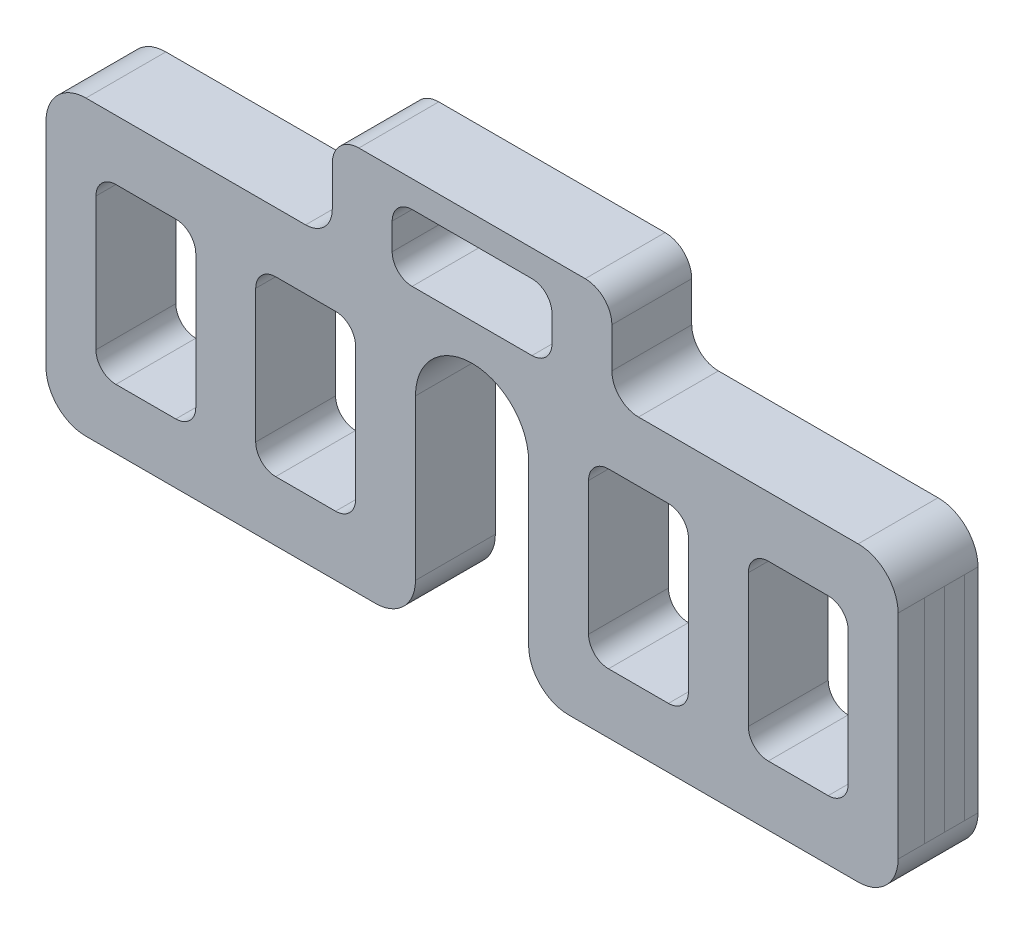
SolidWorks part; units mm, degrees
material "Q235-A"
ref_plane "Front Plane" through (0, 0, 0) normal (0, 0, 1) x (1, 0, 0)
ref_plane "Top Plane" through (0, 0, 0) normal (0, 1, 0) x (1, 0, 0)
ref_plane "Right Plane" through (0, 0, 0) normal (1, 0, 0) x (0, 0, -1)
sketch "Sketch1" plane through (0, 0, 0) normal (0, 0, 1) x (1, 0, 0)
  line L0 (0, -245) -> (0, 245) construction
  line L1 (42.5, 0) -> (320, 0)
  line L3 (45, 220) -> (-45, 220)
  line L4 (60, 235) -> (60, 255)
  line L5 (320, 0) -> (320, 220)
  line L6 (320, 220) -> (125, 220)
  line L7 (42.5, 0) -> (42.5, 150)
  line L8 (-42.5, 0) -> (-42.5, 150)
  line L9 (-320, 0) -> (-320, 220)
  line L10 (45, 270) -> (-45, 270)
  line L11 (-125, 220) -> (-320, 220)
  line L12 (-105, 240) -> (-105, 270)
  line L13 (-42.5, 0) -> (-320, 0)
  line L14 (105, 240) -> (105, 270)
  line L15 (-85, 290) -> (85, 290)
  line L16 (-60, 235) -> (-60, 255)
  line L17 (60, 220) -> (-60, 270) construction
  line L18 (60, 270) -> (-60, 220) construction
  arc A0 (-60, 235) -> (-45, 220) centre (-45, 235) ccw
  arc A1 (45, 220) -> (60, 235) centre (45, 235) ccw
  arc A2 (-42.5, 150) -> (42.5, 150) centre (0, 150) cw
  arc A3 (60, 255) -> (45, 270) centre (45, 255) ccw
  arc A4 (-60, 255) -> (-45, 270) centre (-45, 255) cw
  arc A5 (125, 220) -> (105, 240) centre (125, 240) cw
  arc A6 (-105, 240) -> (-125, 220) centre (-125, 240) cw
  arc A7 (105, 270) -> (85, 290) centre (85, 270) ccw
  arc A8 (-85, 290) -> (-105, 270) centre (-85, 270) ccw
  point P4 (0, 0)
  point P22 (0, 300)
  dimension "D3" = 150
  dimension "D10" = 15
  dimension "D11" = 20
  dimension "D12" = 20
  dimension "D1" = 640
  dimension "D2" = 85
  dimension "D4" = 70
  dimension "D5" = 210
  dimension "D6" = 220
  dimension "D7" = 50
  dimension "D8" = 120
  dimension "D9" = 20
extrude "Boss-Extrude1" add sketch "Sketch1" along normal mid plane 60
sketch "Sketch5" plane through (0, 0, 0) normal (0, 0, 1) x (1, 0, 0)
  line L0 (0, 0) -> (0, 404.8206) construction
  line L1 (-42.5, 0) -> (-42.5, 150) construction
  line L2 (-282.5, 175) -> (-207.5, 175)
  line L3 (-282.5, 175) -> (-282.5, 45)
  line L4 (-282.5, 45) -> (-207.5, 45)
  line L5 (-207.5, 175) -> (-207.5, 45)
  line L6 (-282.5, 175) -> (-207.5, 45) construction
  line L7 (-282.5, 45) -> (-207.5, 175) construction
  line L8 (-162.5, 175) -> (-87.5, 175)
  line L9 (-162.5, 175) -> (-162.5, 45)
  line L10 (-162.5, 45) -> (-87.5, 45)
  line L11 (-87.5, 175) -> (-87.5, 45)
  line L12 (-162.5, 175) -> (-87.5, 45) construction
  line L13 (-162.5, 45) -> (-87.5, 175) construction
  line L14 (-125, 220) -> (-320, 220) construction
  line L15 (-320, 0) -> (-42.5, 0) construction
  point P3 (-245, 110)
  point P8 (-125, 110)
  dimension "D1" = 45
  dimension "D2" = 75
  dimension "D3" = 45
  dimension "D4" = 75
  dimension "D5" = 45
  dimension "D6" = 45
extrude "Cut-Extrude3" cut sketch "Sketch5" against normal through all both and the other way through all
fillet "Fillet2" radius 15 8 edges at (-87.5, 45, 0) (-162.5, 45, 0) (-162.5, 175, 0) (-87.5, 175, 0) (-207.5, 45, 0) (-282.5, 45, 0) (-207.5, 175, 0) (-282.5, 175, 0)
mirror "Mirror3" about plane through (0, 0, 0) normal (1, 0, 0) of "Fillet2", "Cut-Extrude3"
fillet "Fillet3" radius 30 6 edges at (-320, 220, 0) (-320, 0, 0) (-42.5, 0, 0) (320, 220, 0) (320, 0, 0) (42.5, 0, 0)
sketch "Sketch6" plane through (0, 0, 0) normal (1, 0, 0) x (0, 0, -1)
  line L0 (-10, 220) -> (-10, 0)
  line L1 (-30, 220) -> (30, 220) construction
  line L2 (30, 0) -> (-30, 0) construction
  line L3 (5, 220) -> (5, 0)
  line L4 (20, 220) -> (20, 0)
  line L6 (-30, 30) -> (-30, 190) construction
  dimension "D1" = 20
  dimension "D2" = 15
  dimension "D3" = 15
split line "Split Line1"
